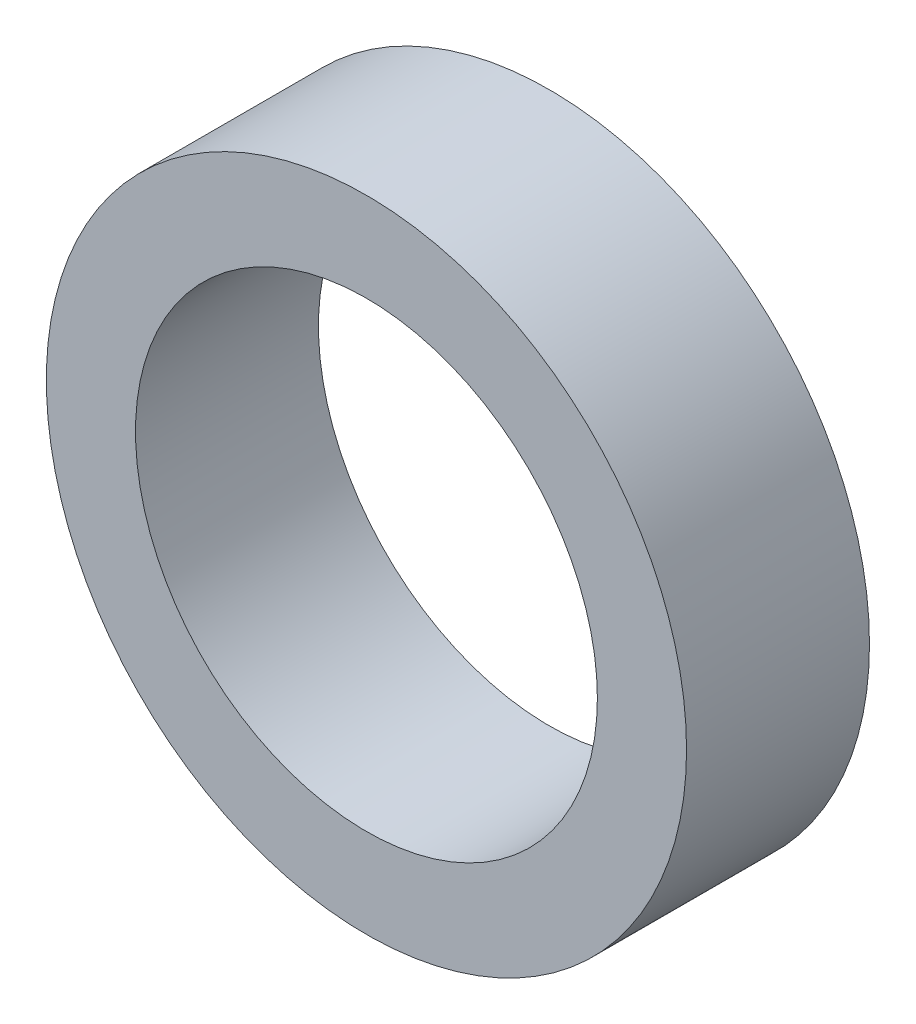
from build123d import *

# Parameters (mm, degrees)
SKETCH1_R           = 14
SKETCH1_R_2         = 10.1
BOSS_EXTRUDE1_DEPTH = 8


with BuildPart() as part:
    # Sketch1 → Boss-Extrude1 (new body)
    with BuildSketch(Plane.XY):
        Circle(SKETCH1_R)
        Circle(SKETCH1_R_2, mode=Mode.SUBTRACT)
    extrude(amount=BOSS_EXTRUDE1_DEPTH)


solid = part.part
